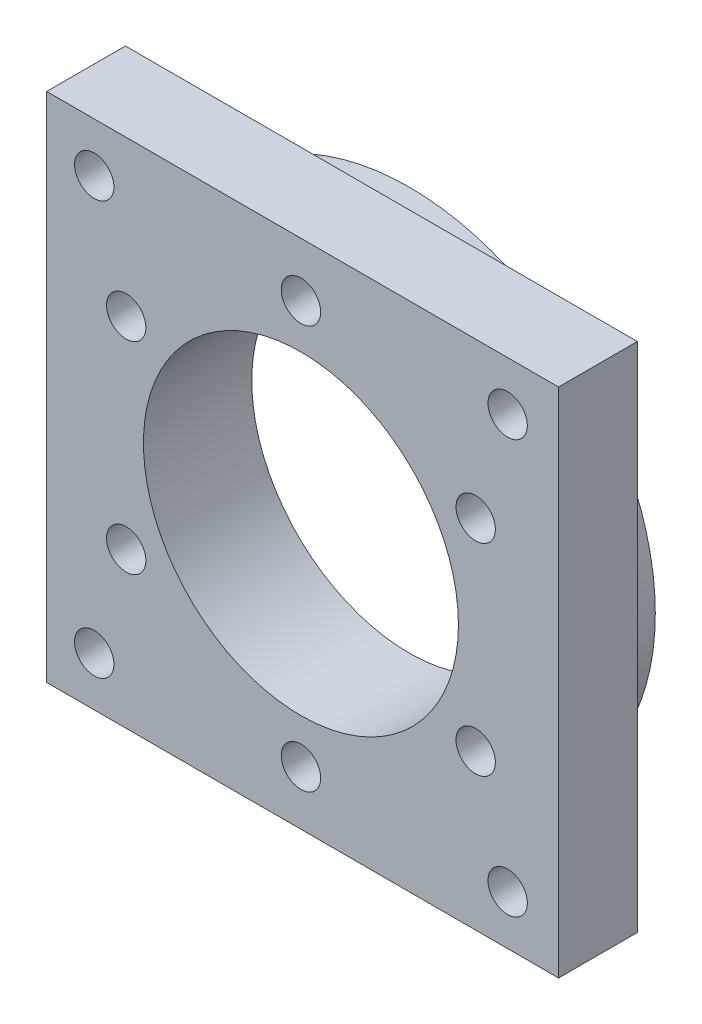
from build123d import *

# Parameters (mm, degrees)
SKETCH1_R           = 25
SKETCH1_R_2         = 16
BOSS_EXTRUDE1_DEPTH = 3
SKETCH2_W           = 52
SKETCH2_H           = 52
SKETCH2_R           = 16
BOSS_EXTRUDE2_DEPTH = 8
SKETCH3_R           = 2
CUT_EXTRUDE1_DEPTH  = 39.495320082
SKETCH4_R           = 2
CUT_EXTRUDE2_DEPTH  = 38.747710768
SKETCH5_R           = 3.5
CUT_EXTRUDE3_DEPTH  = 3


with BuildPart() as part:
    # Sketch1 → Boss-Extrude1 (new body)
    with BuildSketch(Plane.XY):
        Circle(SKETCH1_R)
        Circle(SKETCH1_R_2, mode=Mode.SUBTRACT)
    extrude(amount=BOSS_EXTRUDE1_DEPTH)

    # Sketch2 → Boss-Extrude2 (add)
    with BuildSketch(Plane.XY.offset(3)):
        with Locations((0.170396792, 0)):
            Rectangle(SKETCH2_W, SKETCH2_H)
        Circle(SKETCH2_R, mode=Mode.SUBTRACT)
    extrude(amount=BOSS_EXTRUDE2_DEPTH)

    # Sketch3 → Cut-Extrude1 (cut, through all)
    with BuildSketch(Plane(origin=(0, 0, 0), x_dir=(-1, 0, 0), z_dir=(0, 0, -1))):
        with Locations((0, 20.5)):
            Circle(SKETCH3_R)
        with Locations((17.753520778, 10.25)):
            Circle(SKETCH3_R)
        with Locations((17.753520778, -10.25)):
            Circle(SKETCH3_R)
        with Locations((0, -20.5)):
            Circle(SKETCH3_R)
        with Locations((-17.753520778, -10.25)):
            Circle(SKETCH3_R)
        with Locations((-17.753520778, 10.25)):
            Circle(SKETCH3_R)
    extrude(amount=-CUT_EXTRUDE1_DEPTH, mode=Mode.SUBTRACT)

    # Sketch4 → Cut-Extrude2 (cut, through all)
    with BuildSketch(Plane(origin=(0, 0, 3), x_dir=(-1, 0, 0), z_dir=(0, 0, -1))):
        with Locations((-21, 21)):
            Circle(SKETCH4_R)
        with Locations(Location((21, 21, 0), (0, 0, 180))):
            Circle(SKETCH4_R)
        with Locations((21, -21)):
            Circle(SKETCH4_R)
        with Locations(Location((-21, -21, 0), (0, 0, 180))):
            Circle(SKETCH4_R)
    extrude(amount=-CUT_EXTRUDE2_DEPTH, mode=Mode.SUBTRACT)

    # Sketch5 → Cut-Extrude3 (cut)
    with BuildSketch(Plane(origin=(0, 0, 0), x_dir=(-1, 0, 0), z_dir=(0, 0, -1))):
        with Locations((0, 20.5)):
            Circle(SKETCH5_R)
        with Locations((17.753520778, 10.25)):
            Circle(SKETCH5_R)
        with Locations((17.753520778, -10.25)):
            Circle(SKETCH5_R)
        with Locations((0, -20.5)):
            Circle(SKETCH5_R)
        with Locations((-17.753520778, -10.25)):
            Circle(SKETCH5_R)
        with Locations((-17.753520778, 10.25)):
            Circle(SKETCH5_R)
    extrude(amount=-CUT_EXTRUDE3_DEPTH, mode=Mode.SUBTRACT)


solid = part.part
